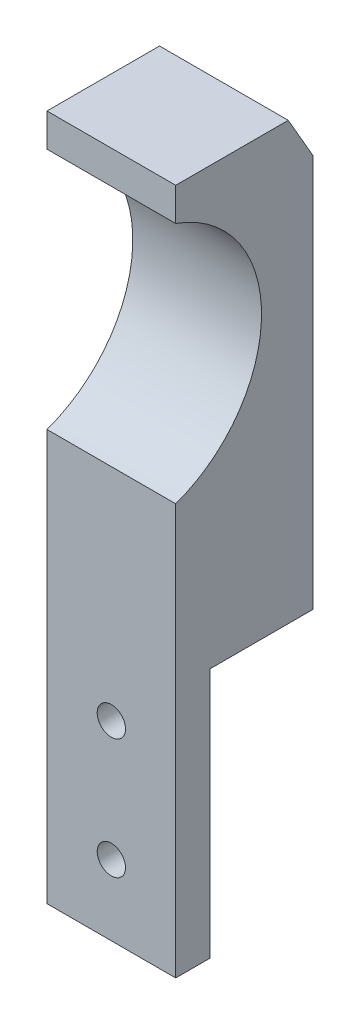
from build123d import *

# Parameters (mm, degrees)
SKETCH1_W             = 15
SKETCH1_H             = 80
BOSS_EXTRUDE1_DEPTH   = 16
SKETCH2_W             = 12
SKETCH2_H             = 29.2
CUT_EXTRUDE1_DEPTH    = 46.617978912
M4_TAPPED_HOLE1_D     = 3.3
M4_TAPPED_HOLE1_DEPTH = 22.25
M4_TAPPED_HOLE1_TIP   = 0.991420021
CHAMFER1_SIZE         = 5
CHAMFER1_SIZE2        = 2.886751346
SKETCH6_R             = 15
CUT_EXTRUDE2_DEPTH    = 46.617978912


with BuildPart() as part:
    # Sketch1 → Boss-Extrude1 (new body)
    with BuildSketch(Plane.XY):
        Rectangle(SKETCH1_W, SKETCH1_H)
    extrude(amount=BOSS_EXTRUDE1_DEPTH)

    # Sketch2 → Cut-Extrude1 (cut, through all)
    with BuildSketch(Plane(origin=(7.5, 0, 0), x_dir=(0, 0, -1), z_dir=(1, 0, 0))):
        with Locations((-6, -25.4)):
            Rectangle(SKETCH2_W, SKETCH2_H)
    extrude(amount=-CUT_EXTRUDE1_DEPTH, mode=Mode.SUBTRACT)

    # M4 Tapped Hole1
    with Locations(Plane(origin=(0, 0, 12), x_dir=(-1, 0, 0), z_dir=(0, 0, -1))):
        with Locations((0, -17.8), (0, -31.8)):
            Hole(M4_TAPPED_HOLE1_D / 2, depth=M4_TAPPED_HOLE1_DEPTH)
            with Locations((0, 0, -(M4_TAPPED_HOLE1_DEPTH + M4_TAPPED_HOLE1_TIP / 2))):  # 118° drill point
                Cone(0, M4_TAPPED_HOLE1_D / 2, M4_TAPPED_HOLE1_TIP, mode=Mode.SUBTRACT)

    # Chamfer1
    chamfer1_edges = [part.edges().sort_by_distance(p)[0] for p in [
        (0, 40, 0),
    ]]
    chamfer1_side = [part.faces().sort_by_distance(p)[0] for p in [
        (0, 14.6, 0),
    ]]
    chamfer(chamfer1_edges, length=CHAMFER1_SIZE, length2=CHAMFER1_SIZE2, reference=chamfer1_side[0])

    # Sketch6 → Cut-Extrude2 (cut, through all)
    with BuildSketch(Plane(origin=(7.5, 0, 0), x_dir=(0, 0, -1), z_dir=(1, 0, 0))):
        with Locations((-21, 22)):
            Circle(SKETCH6_R)
    extrude(amount=-CUT_EXTRUDE2_DEPTH, mode=Mode.SUBTRACT)


solid = part.part
